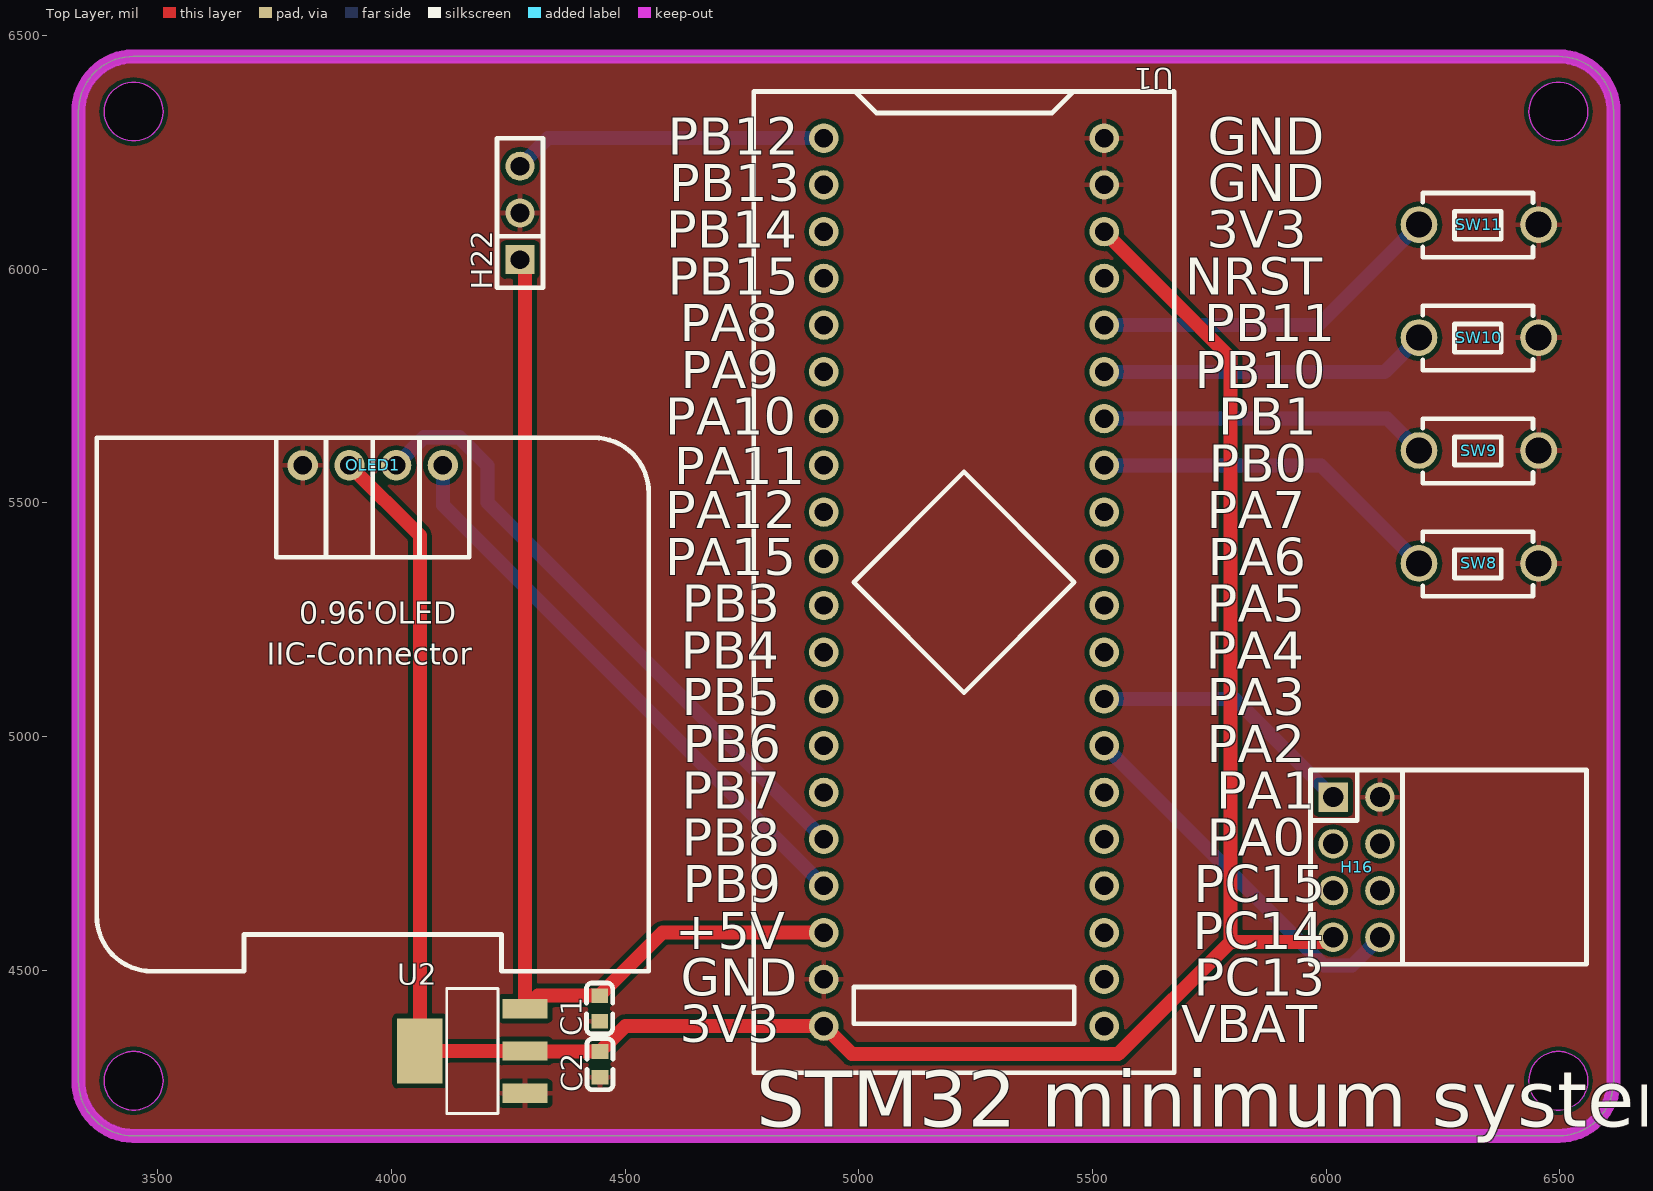
[diagram p0: Top Layer view]
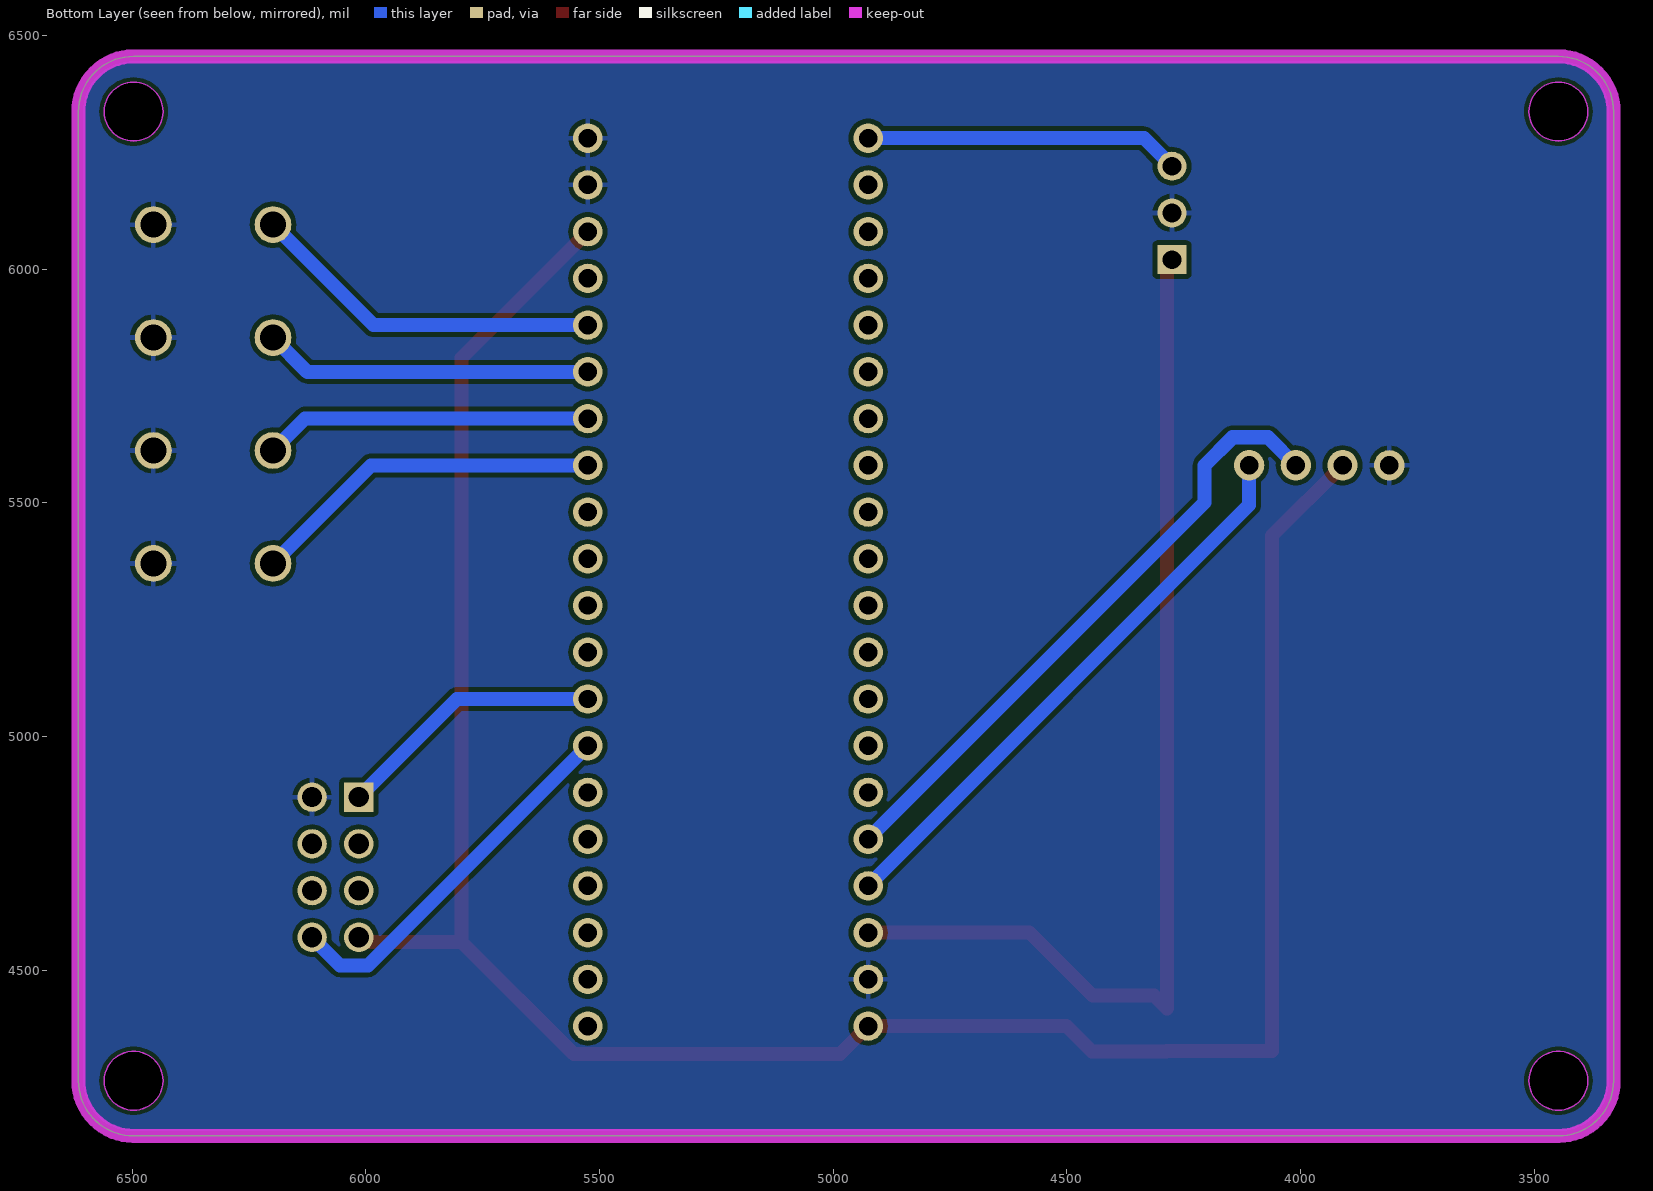
[diagram p1: Bottom Layer view, seen from below]
# Altium PCB MISC89072.pcbdoc
Units mil, origin at the board's own origin, x right, y up, seen from the top; angles counter-clockwise.
Board outline 3285 x 2310 mil, 2 copper layers (Top Layer, Bottom Layer), stack 62.206 mil thick; 11 components, 37 nets, 71 pads, 0 vias.

## Layer stack, top to bottom
Top Solder Mask Layer: solder mask 0.394, Dk 3.3
Top Layer: signal copper 1.379
Dielectric1: surface 59.449, FR4, Dk 4.5
Bottom Layer: signal copper 1.378
Bottom Solder Mask Layer: solder mask 0.394, Dk 3.3

## Board outline
3448.11,6455 ccw(c3448.11,6336.89) 3330,6336.89 3330,4263.11 ccw(c3448.11,4263.11) 3448.11,4145 6496.89,4145 ccw(c6496.89,4263.11) 6615,4263.11 6615,6336.89 ccw(c6496.89,6336.89) 6496.89,6455
cut-out: 3511.1,4263.11 cw(c3448.11,4263.11) 3385.12,4263.11 cw(c3448.11,4263.11)
cut-out: 6559.88,4263.11 cw(c6496.89,4263.11) 6433.9,4263.11 cw(c6496.89,4263.11)
cut-out: 6559.88,6336.89 cw(c6496.89,6336.89) 6433.9,6336.89 cw(c6496.89,6336.89)
cut-out: 3511.1,6336.89 cw(c3448.11,6336.89) 3385.12,6336.89 cw(c3448.11,6336.89)

## Design rules (kind name [scope] priority, off if disabled: settings)
BoardOutlineClearance copperThickness2oz_1 [All] p2 off: genericclearance=7.99 ignorepadtopadclearanceinfootprint=FALSE except(0: Arc-SplitContinuation Track-SplitContinuation SMDPad-SplitContinuation THPad-SplitContinuation Via-SplitContinuation Fill-SplitContinuation Region-SplitContinuation Poly-SplitContinuation Text-SplitContinuation Hole-SplitContinuation; 5.98: Arc-CutoutEdge Track-CutoutEdge SMDPad-CutoutEdge THPad-CutoutEdge Via-CutoutEdge Text-CutoutEdge; 6.89: Hole-OutlineEdge Hole-CutoutEdge; 10: Poly-OutlineEdge Poly-CutoutEdge; 11.81: Arc-OutlineEdge Track-OutlineEdge SMDPad-OutlineEdge THPad-OutlineEdge Via-OutlineEdge Fill-OutlineEdge Region-OutlineEdge Text-OutlineEdge Fill-CutoutEdge Region-CutoutEdge)
BoardOutlineClearance Plane_innerPlane_1 [All] p4 off: genericclearance=4.02 ignorepadtopadclearanceinfootprint=FALSE except(0: Arc-SplitContinuation Track-SplitContinuation SMDPad-SplitContinuation THPad-SplitContinuation Via-SplitContinuation Fill-SplitContinuation Region-SplitContinuation Poly-SplitContinuation Text-SplitContinuation Hole-SplitContinuation; 5.98: Arc-CutoutEdge Track-CutoutEdge SMDPad-CutoutEdge THPad-CutoutEdge Via-CutoutEdge Text-CutoutEdge; 6.89: Hole-OutlineEdge Hole-CutoutEdge; 10: Poly-OutlineEdge Poly-CutoutEdge; 11.81: Arc-OutlineEdge Track-OutlineEdge SMDPad-OutlineEdge THPad-OutlineEdge Via-OutlineEdge Fill-OutlineEdge Region-OutlineEdge Text-OutlineEdge Fill-CutoutEdge Region-CutoutEdge)
BoardOutlineClearance Copper_copperRegion_1 [All] p6 off: genericclearance=4.02 ignorepadtopadclearanceinfootprint=FALSE except(0: Arc-SplitContinuation Track-SplitContinuation SMDPad-SplitContinuation THPad-SplitContinuation Via-SplitContinuation Fill-SplitContinuation Region-SplitContinuation Poly-SplitContinuation Text-SplitContinuation Hole-SplitContinuation; 5.98: Arc-CutoutEdge Track-CutoutEdge SMDPad-CutoutEdge THPad-CutoutEdge Via-CutoutEdge Text-CutoutEdge; 6.89: Hole-OutlineEdge Hole-CutoutEdge; 10: Poly-OutlineEdge Poly-CutoutEdge; 11.81: Arc-OutlineEdge Track-OutlineEdge SMDPad-OutlineEdge THPad-OutlineEdge Via-OutlineEdge Fill-OutlineEdge Region-OutlineEdge Text-OutlineEdge Fill-CutoutEdge Region-CutoutEdge)
BoardOutlineClearance copperThickness1oz_1 [All] p8: genericclearance=4.02 ignorepadtopadclearanceinfootprint=FALSE except(0: Arc-SplitContinuation Track-SplitContinuation SMDPad-SplitContinuation THPad-SplitContinuation Via-SplitContinuation Fill-SplitContinuation Region-SplitContinuation Poly-SplitContinuation Text-SplitContinuation Hole-SplitContinuation; 5.98: Arc-CutoutEdge Track-CutoutEdge SMDPad-CutoutEdge THPad-CutoutEdge Via-CutoutEdge Text-CutoutEdge; 6.89: Hole-OutlineEdge Hole-CutoutEdge; 10: Poly-OutlineEdge Poly-CutoutEdge; 11.81: Arc-OutlineEdge Track-OutlineEdge SMDPad-OutlineEdge THPad-OutlineEdge Via-OutlineEdge Fill-OutlineEdge Region-OutlineEdge Text-OutlineEdge Fill-CutoutEdge Region-CutoutEdge)
Clearance copperThickness2oz [All] p1 off: gap=7.99 ignorepadtopadclearanceinfootprint=FALSE except(5.98: SMDPad-Track SMDPad-SMDPad THPad-Track SMDPad-THPad THPad-THPad Track-Via SMDPad-Via THPad-Via Via-Via Fill-SMDPad Region-SMDPad Fill-THPad Region-THPad Fill-Via Region-Via Fill-Fill Fill-Region Region-Region Arc-Track Arc-SMDPad Arc-THPad Arc-Via Fill-Arc Region-Arc Arc-Arc Text-Track SMDPad-Text Text-THPad Text-Via Fill-Text Region-Text Arc-Text Text-Text; 6.89: Hole-Track Hole-SMDPad Hole-THPad Hole-Via Fill-Hole Region-Hole Hole-Arc Hole-Text; 10: Poly-Track Poly-SMDPad Poly-THPad Poly-Via Poly-Fill Poly-Region Poly-Poly Poly-Arc Poly-Text Poly-Hole; 11.81: Fill-Track Region-Track)
Clearance Plane_innerPlane [All] p3 off: gap=4.02 ignorepadtopadclearanceinfootprint=FALSE except(5.98: SMDPad-Track SMDPad-SMDPad THPad-Track SMDPad-THPad THPad-THPad Track-Via SMDPad-Via THPad-Via Via-Via Fill-SMDPad Region-SMDPad Fill-THPad Region-THPad Fill-Via Region-Via Fill-Fill Fill-Region Region-Region Arc-Track Arc-SMDPad Arc-THPad Arc-Via Fill-Arc Region-Arc Arc-Arc Text-Track SMDPad-Text Text-THPad Text-Via Fill-Text Region-Text Arc-Text Text-Text; 6.89: Hole-Track Hole-SMDPad Hole-THPad Hole-Via Fill-Hole Region-Hole Hole-Arc Hole-Text; 10: Poly-Track Poly-SMDPad Poly-THPad Poly-Via Poly-Fill Poly-Region Poly-Poly Poly-Arc Poly-Text Poly-Hole; 11.81: Fill-Track Region-Track)
Clearance Copper_copperRegion [All] p5 off: gap=4.02 ignorepadtopadclearanceinfootprint=FALSE except(5.98: SMDPad-Track SMDPad-SMDPad THPad-Track SMDPad-THPad THPad-THPad Track-Via SMDPad-Via THPad-Via Via-Via Fill-SMDPad Region-SMDPad Fill-THPad Region-THPad Fill-Via Region-Via Fill-Fill Fill-Region Region-Region Arc-Track Arc-SMDPad Arc-THPad Arc-Via Fill-Arc Region-Arc Arc-Arc Text-Track SMDPad-Text Text-THPad Text-Via Fill-Text Region-Text Arc-Text Text-Text; 6.89: Hole-Track Hole-SMDPad Hole-THPad Hole-Via Fill-Hole Region-Hole Hole-Arc Hole-Text; 10: Poly-Track Poly-SMDPad Poly-THPad Poly-Via Poly-Fill Poly-Region Poly-Poly Poly-Arc Poly-Text Poly-Hole; 11.81: Fill-Track Region-Track)
Clearance copperThickness1oz [All] p7: gap=4.02 ignorepadtopadclearanceinfootprint=FALSE except(5.98: SMDPad-Track SMDPad-SMDPad THPad-Track SMDPad-THPad THPad-THPad Track-Via SMDPad-Via THPad-Via Via-Via Fill-SMDPad Region-SMDPad Fill-THPad Region-THPad Fill-Via Region-Via Fill-Fill Fill-Region Region-Region Arc-Track Arc-SMDPad Arc-THPad Arc-Via Fill-Arc Region-Arc Arc-Arc Text-Track SMDPad-Text Text-THPad Text-Via Fill-Text Region-Text Arc-Text Text-Text; 6.89: Hole-Track Hole-SMDPad Hole-THPad Hole-Via Fill-Hole Region-Hole Hole-Arc Hole-Text; 10: Poly-Track Poly-SMDPad Poly-THPad Poly-Via Poly-Fill Poly-Region Poly-Poly Poly-Arc Poly-Text Poly-Hole; 11.81: Fill-Track Region-Track)
DiffPairsRouting differentialPair [All] p1: maxlimit=6 minlimit=6 mostfreqgap=6 toplayer_minwidth=5 toplayer_prefwidth=10 toplayer_maxwidth=100 toplayer_mingap=6 toplayer_prefgap=6 toplayer_maxgap=6 bottomlayer_minwidth=5 bottomlayer_prefwidth=10 bottomlayer_maxwidth=100 bottomlayer_mingap=6 bottomlayer_prefgap=6 bottomlayer_maxgap=6 maxuncoupledlength=10
HoleToHoleClearance otherClearance [All] p1: gap=11.81 allowstackedmicrovias=TRUE
Length netLength [All] p1: minlimit=0 maxlimit=0
PasteMaskExpansion pasteMaskExpansion [All] p1: expansion=0
PlaneConnect innerPlane [All] p1: planeconnectstyle=Relief reliefexpansion=20 reliefentries=4 reliefconductorwidth=10 reliefairgap=10
PolygonConnect copperRegion [All] p1: connectstyle=Relief reliefconductorwidth=10 reliefentries=4 polygonreliefangle="90 Angle" airgapwidth=10 via.connectstyle=Relief via.reliefconductorwidth=10 via.reliefentries=4 via.polygonreliefangle="90 Angle" via.airgapwidth=10
RoutingVias viaSize [All] p1: holewidth=12.01 width=24.02 viastyle="Through Hole" minholewidth=11.81 minwidth=19.68 maxholewidth=248.03 maxwidth=393.7
SolderMaskExpansion solderMaskExpansion [IsVia] p1: expansion=-1000 istentingtop=TRUE
SolderMaskExpansion solderMaskExpansion [All] p2: expansion=2.01 istentingtop=FALSE
Width copperThickness2oz_2 [All] p1 off: maxlimit=100 minlimit=8 preferedwidth=10
Width copperThickness1oz_2 [All] p2: maxlimit=100 minlimit=5 preferedwidth=30

## Components (designator, comment, footprint, x,y, rotation, side; value= is the part's Value field where it differs from the comment)
C1 "100nF" C0603 4445.15,4417.73 r90 top
C2 "100nF" C0603 4446.16,4298.32 r90 top
H16 "" HDR-TH_8P-P2.54-V-F-R2-C4-S2.54-1 6065,4720 r270 top
H22 "" HDR-TH_3P-P2.54-V-F 4275,6120 r90 top
OLED1 "" 0.96OLED_4P 3960,5580 r0 top
SW8 "" Key_TH_3.5x6x4.3 6320,5370 r0 top
SW9 "" Key_TH_3.5x6x4.3 6320,5611.67 r0 top
SW10 "" Key_TH_3.5x6x4.3 6320,5853.33 r0 top
SW11 "" Key_TH_3.5x6x4.3 6320,6095 r0 top
U1 "STM32F103C8T6-Card" CONN-TH_L53.3-W22.9_STM32F103C8T6-CARD 5225,5330 r270 top
U2 "AMS1117-5.0" SOT-223_L6.5-W3.5-P2.30-LS7.0-BR 4173.03,4326.87 r0 top

## Footprints (in the part's own frame and the unit in brackets; to place one, negate y for a bottom-side part, rotate by r counter-clockwise, add the part's x,y. Pads: shape width x height; smd on the part's side, far side on the other; paste and mask are expansions set on the pad)
0.96OLED_4P [mm]
  round 1.65 hole 1 copper offset 0,0: 1(-3.81,-0.001) 2(-1.27,0.002) 3(1.27,0.002) 4(3.81,0.002)
  silkscreen extent -15,-27.5 15,1.5
C0603 [mm]
  rect 0.8x0.9 smd: 1(-0.7,0) 2(0.7,0)
  silkscreen extent -1.39,-0.71 1.39,0.71
CONN-TH_L53.3-W22.9_STM32F103C8T6-CARD [mm]
  round 1.6 hole 1: 1(-24.13,-7.62) 2(-21.59,-7.62) 3(-19.05,-7.62) 4(-16.51,-7.62) 5(-13.97,-7.62) 6(-11.43,-7.62) 7(-8.89,-7.62) 8(-6.35,-7.62) 9(-3.81,-7.62) 10(-1.27,-7.62) 11(1.27,-7.62) 12(3.81,-7.62) 13(6.35,-7.62) 14(8.89,-7.62) 15(11.43,-7.62) 16(13.97,-7.62) 17(16.51,-7.62) 18(19.05,-7.62) 19(21.59,-7.62) 20(24.13,-7.62) 21(24.13,7.62) 22(21.59,7.62) 23(19.05,7.62) 24(16.51,7.62) 25(13.97,7.62) 26(11.43,7.62) 27(8.89,7.62) 28(6.35,7.62) 29(3.81,7.62) 30(1.27,7.62) 31(-1.27,7.62) 32(-3.81,7.62) 33(-6.35,7.62) 34(-8.89,7.62) 35(-11.43,7.62) 36(-13.97,7.62) 37(-16.51,7.62) 38(-19.05,7.62) 39(-21.59,7.62) 40(-24.13,7.62)
  silkscreen extent -26.67,-11.43 26.67,11.43
HDR-TH_3P-P2.54-V-F [mil]
  rect 62x62 hole 40.16: 1(-100,0)
  round 62 hole 40.16: 2(0,0) 3(100,0)
  silkscreen extent -160,-49 160,49
HDR-TH_8P-P2.54-V-F-R2-C4-S2.54-1 [mm]
  rect 1.6x1.6 hole 1.1: 1(-3.81,-1.27)
  round 1.6 hole 1.1: 2(-3.81,1.27) 3(-1.27,-1.27) 4(-1.27,1.27) 5(1.27,-1.27) 6(1.27,1.27) 7(3.81,-1.27) 8(3.81,1.27)
  silkscreen extent -5.28,-2.5 5.28,12.5
Key_TH_3.5x6x4.3 [mil]
  round 78.7 hole 55.1 paste+0 mask+2: A(-121.44,0) B(134.46,0)
  silkscreen extent -114,-70 123,68
SOT-223_L6.5-W3.5-P2.30-LS7.0-BR [mm]
  rect 2.465x1.05 smd: 1(2.857,-2.3) 2(2.857,0) 3(2.857,2.3)
  rect 2.465x3.54 smd: 4(-2.857,0)
  silkscreen extent -1.4,-3.4 1.4,3.4

## Nets (pads, with @x,y where several pads share a name; then routed paths per layer and width w, separated by ;. In a path a pad name is that pad's centre, name@x,y a point inside that pad or via, vN(x,y) a via of type N, cw(c..) or ccw(c..) an arc to the next point about the centre after c; other vN are vias at no path point)
+5V: C1.2 H22.1 U1.18 U2.3 | length 2313.8
  Top Layer w30: H22.1 4285.53,6009.47 U2.3 4313.4,4445.29 C1.2 4579.87,4580 U1.18
GND: C1.1 C2.1 H16.2 H22.2 OLED1.1 SW8.B SW9.B SW10.B SW11.B U1.19 U1.39 U1.40 U2.1
NRST: U1.37
PA0: U1.25
PA1: U1.26
PA2: H16.8 U1.27 | length 809.5
  Bottom Layer w30: U1.27 5995,4510 6055,4510 H16.8
PA3: H16.1 U1.28 | length 577
  Bottom Layer w30: U1.28 5805,5080 H16.1
PA4: U1.29
PA5: U1.30
PA6: U1.31
PA7: U1.32
PA8: U1.5
PA9: U1.6
PA10: U1.7
PA11: U1.8
PA12: U1.9
PA15: U1.10
PB0: SW8.A U1.33 | length 760.5
  Bottom Layer w30: U1.33 5988.56,5580 SW8.A
PB1: SW9.A U1.34 | length 701.9
  Bottom Layer w30: U1.34 6130.23,5680 SW9.A
PB3: U1.11
PB4: U1.12
PB5: U1.13
PB6: U1.14
PB7: U1.15
PB8: OLED1.3 U1.16 | length 1343
  Bottom Layer w30: OLED1.3@4010,5580.05 4070,5640.05 4145,5640.05 4205,5580.05 4205,5500 U1.16
PB9: OLED1.4 U1.17 | length 1237.6
  Bottom Layer w30: OLED1.4@4110,5580.05 4110,5495 U1.17
PB10: SW10.A U1.35 | length 703.9
  Bottom Layer w30: U1.35 6125.22,5780 SW10.A
PB11: SW11.A U1.36 | length 762.6
  Bottom Layer w30: U1.36 5983.56,5880 SW11.A
PB12: H22.3 U1.1 | length 674.9
  Bottom Layer w30: H22.3 4335,6280 U1.1
PB13: U1.2
PB14: U1.3
PB15: U1.4
PC13: U1.22
PC14: U1.23
PC15: U1.24
VBAT: U1.21
VCC: C2.2 H16.7 OLED1.2 U1.20 U1.38 U2.2 U2.4 | length 5053.1
  Top Layer w30: OLED1.2@3910,5580.05 4060.53,5429.52 U2.4 U2.2 4286.51,4325.88 C2.2 4500.28,4380 U1.20 4985,4320 5555,4320 5795,4560 ; U1.38 5795,5810 5795,4560 ; H16.7 6005,4560 5795,4560
pads on no net: H16.3 H16.4 H16.5 H16.6

## Polygon pours and split planes (outlines as drawn)
GND on Bottom Layer (solid, remove dead copper, pour order 2): 3100,7165 3100,3000 7275,3000 7275,7165
GND on Top Layer (solid, remove dead copper, pour order 0): 3000,7145 3000,3075 7385,3075 7385,7145

## Keep-outs
Board Outline Layer:
  region: 3511.1,4263.11 cw(c3448.11,4263.11) 3385.12,4263.11 cw(c3448.11,4263.11)
  circle w0.1: c3448.11,4263.11 r62.99
  region: 3511.1,4263.11 3510.71,4256.06 3509.52,4249.09 3507.57,4242.31 3504.86,4235.78 3501.45,4229.6 3497.36,4223.84 3492.65,4218.57 3487.39,4213.86 3481.62,4209.77 3475.44,4206.36 3468.92,4203.65 3462.13,4201.7 3455.16,4200.51 3448.11,4200.12 3441.06,4200.51 3434.09,4201.7 3427.31,4203.65 3420.78,4206.36 3414.6,4209.77 3408.84,4213.86 3403.57,4218.57 3398.86,4223.84 3394.77,4229.6 3391.36,4235.78 3388.65,4242.31 3386.7,4249.09 3385.51,4256.06 3385.12,4263.11 3385.51,4270.16 3386.7,4277.13 3388.65,4283.92 3391.36,4290.44 3394.77,4296.62 3398.86,4302.39 3403.57,4307.65 3408.84,4312.36 3414.6,4316.45 3420.78,4319.86 3427.31,4322.57 3434.09,4324.52 3441.06,4325.71 3448.11,4326.1 3455.16,4325.71 3462.13,4324.52 3468.92,4322.57 3475.44,4319.86 3481.62,4316.45 3487.39,4312.36 3492.65,4307.65 3497.36,4302.39 3501.45,4296.62 3504.86,4290.44 3507.57,4283.92 3509.52,4277.13 3510.71,4270.16
  region: 6559.88,4263.11 cw(c6496.89,4263.11) 6433.9,4263.11 cw(c6496.89,4263.11)
  circle w0.1: c6496.89,4263.11 r62.99
  region: 6559.88,4263.11 6559.49,4256.06 6558.3,4249.09 6556.35,4242.31 6553.64,4235.78 6550.23,4229.6 6546.14,4223.84 6541.43,4218.57 6536.16,4213.86 6530.4,4209.77 6524.22,4206.36 6517.69,4203.65 6510.91,4201.7 6503.94,4200.51 6496.89,4200.12 6489.84,4200.51 6482.87,4201.7 6476.08,4203.65 6469.56,4206.36 6463.38,4209.77 6457.61,4213.86 6452.35,4218.57 6447.64,4223.84 6443.55,4229.6 6440.14,4235.78 6437.43,4242.31 6435.48,4249.09 6434.29,4256.06 6433.9,4263.11 6434.29,4270.16 6435.48,4277.13 6437.43,4283.92 6440.14,4290.44 6443.55,4296.62 6447.64,4302.39 6452.35,4307.65 6457.61,4312.36 6463.38,4316.45 6469.56,4319.86 6476.08,4322.57 6482.87,4324.52 6489.84,4325.71 6496.89,4326.1 6503.94,4325.71 6510.91,4324.52 6517.69,4322.57 6524.22,4319.86 6530.4,4316.45 6536.16,4312.36 6541.43,4307.65 6546.14,4302.39 6550.23,4296.62 6553.64,4290.44 6556.35,4283.92 6558.3,4277.13 6559.49,4270.16
  region: 6559.88,6336.89 cw(c6496.89,6336.89) 6433.9,6336.89 cw(c6496.89,6336.89)
  circle w0.1: c6496.89,6336.89 r62.99
  region: 6559.88,6336.89 6559.49,6329.84 6558.3,6322.87 6556.35,6316.08 6553.64,6309.56 6550.23,6303.38 6546.14,6297.61 6541.43,6292.35 6536.16,6287.64 6530.4,6283.55 6524.22,6280.14 6517.69,6277.43 6510.91,6275.48 6503.94,6274.29 6496.89,6273.9 6489.84,6274.29 6482.87,6275.48 6476.08,6277.43 6469.56,6280.14 6463.38,6283.55 6457.61,6287.64 6452.35,6292.35 6447.64,6297.61 6443.55,6303.38 6440.14,6309.56 6437.43,6316.08 6435.48,6322.87 6434.29,6329.84 6433.9,6336.89 6434.29,6343.94 6435.48,6350.91 6437.43,6357.69 6440.14,6364.22 6443.55,6370.4 6447.64,6376.16 6452.35,6381.43 6457.61,6386.14 6463.38,6390.23 6469.56,6393.64 6476.08,6396.35 6482.87,6398.3 6489.84,6399.49 6496.89,6399.88 6503.94,6399.49 6510.91,6398.3 6517.69,6396.35 6524.22,6393.64 6530.4,6390.23 6536.16,6386.14 6541.43,6381.43 6546.14,6376.16 6550.23,6370.4 6553.64,6364.22 6556.35,6357.69 6558.3,6350.91 6559.49,6343.94
  region: 3511.1,6336.89 cw(c3448.11,6336.89) 3385.12,6336.89 cw(c3448.11,6336.89)
  circle w0.1: c3448.11,6336.89 r62.99
  region: 3511.1,6336.89 3510.71,6329.84 3509.52,6322.87 3507.57,6316.08 3504.86,6309.56 3501.45,6303.38 3497.36,6297.61 3492.65,6292.35 3487.39,6287.64 3481.62,6283.55 3475.44,6280.14 3468.92,6277.43 3462.13,6275.48 3455.16,6274.29 3448.11,6273.9 3441.06,6274.29 3434.09,6275.48 3427.31,6277.43 3420.78,6280.14 3414.6,6283.55 3408.84,6287.64 3403.57,6292.35 3398.86,6297.61 3394.77,6303.38 3391.36,6309.56 3388.65,6316.08 3386.7,6322.87 3385.51,6329.84 3385.12,6336.89 3385.51,6343.94 3386.7,6350.91 3388.65,6357.69 3391.36,6364.22 3394.77,6370.4 3398.86,6376.16 3403.57,6381.43 3408.84,6386.14 3414.6,6390.23 3420.78,6393.64 3427.31,6396.35 3434.09,6398.3 3441.06,6399.49 3448.11,6399.88 3455.16,6399.49 3462.13,6398.3 3468.92,6396.35 3475.44,6393.64 3481.62,6390.23 3487.39,6386.14 3492.65,6381.43 3497.36,6376.16 3501.45,6370.4 3504.86,6364.22 3507.57,6357.69 3509.52,6350.91 3510.71,6343.94
  lines w30: 3330,4263.11 3330,6336.89 cw(c3448.11,6336.89) 3448.11,6455 6496.89,6455 cw(c6496.89,6336.89) 6615,6336.89 6615,4263.11 cw(c6496.89,4263.11) 6496.89,4145 3448.11,4145 cw(c3448.11,4263.11) 3330,4263.11

## Silkscreen, mask and mechanical layers (free items; w line width, h text height)
Top Silkscreen Layer:
  text "PB12" at 4590.64,6245 h80
  text "GND" at 5746.65,6245 h80
  text "PB13" at 4593.85,6145 h80
  text "GND" at 5746.65,6145 h80
  text "PB14" at 4588.34,6045 h80
  text "3V3" at 5744.45,6045 h80
  text "PB15" at 4590.64,5945 h80
  text "NRST" at 5698.65,5945 h80
  text "PA8" at 4616.24,5845 h80
  text "PB11" at 5739.05,5845 h80
  text "PA9" at 4618.44,5745 h80
  text "PB10" at 5718.85,5745 h80
  text "PA10" at 4586.14,5645 h80
  text "PB1" at 5769.15,5645 h80
  text "PB0" at 5748.95,5545 h80
  text "PA11" at 4604.55,5540 h80
  text "PA12" at 4586.14,5445 h80
  text "PA7" at 5744.45,5445 h80
  text "PA15" at 4586.14,5345 h80
  text "PA6" at 5746.65,5345 h80
  text "PB3" at 4620.74,5245 h80
  text "PA5" at 5744.45,5245 h80
  text "PB4" at 4618.44,5145 h80
  text "PA4" at 5742.15,5145 h80
  text "PB5" at 4620.74,5045 h80
  text "PA3" at 5744.45,5045 h80
  text "PB6" at 4622.94,4945 h80
  text "PA2" at 5744.45,4945 h80
  text "PB7" at 4620.74,4845 h80
  text "PA1" at 5764.65,4845 h80
  text "PB8" at 4620.74,4745 h80
  text "PA0" at 5744.45,4745 h80
  text "PB9" at 4622.94,4645 h80
  text "PC15" at 5716.55,4645 h80
  text "+5V" at 4607.24,4545 h80
  text "PC14" at 5714.25,4545 h80
  text "GND" at 4618.44,4445 h80
  text "PC13" at 5716.55,4445 h80
  text "3V3" at 4616.24,4345 h80
  text "VBAT" at 5689.65,4345 h80
  text "STM32 minimum system" at 4780,4165 h120
Mechanical Layer:
  circle w0.1: c3448.11,4263.11 r62.99
  circle w0.1: c6496.89,4263.11 r62.99
  circle w0.1: c6496.89,6336.89 r62.99
  circle w0.1: c3448.11,6336.89 r62.99